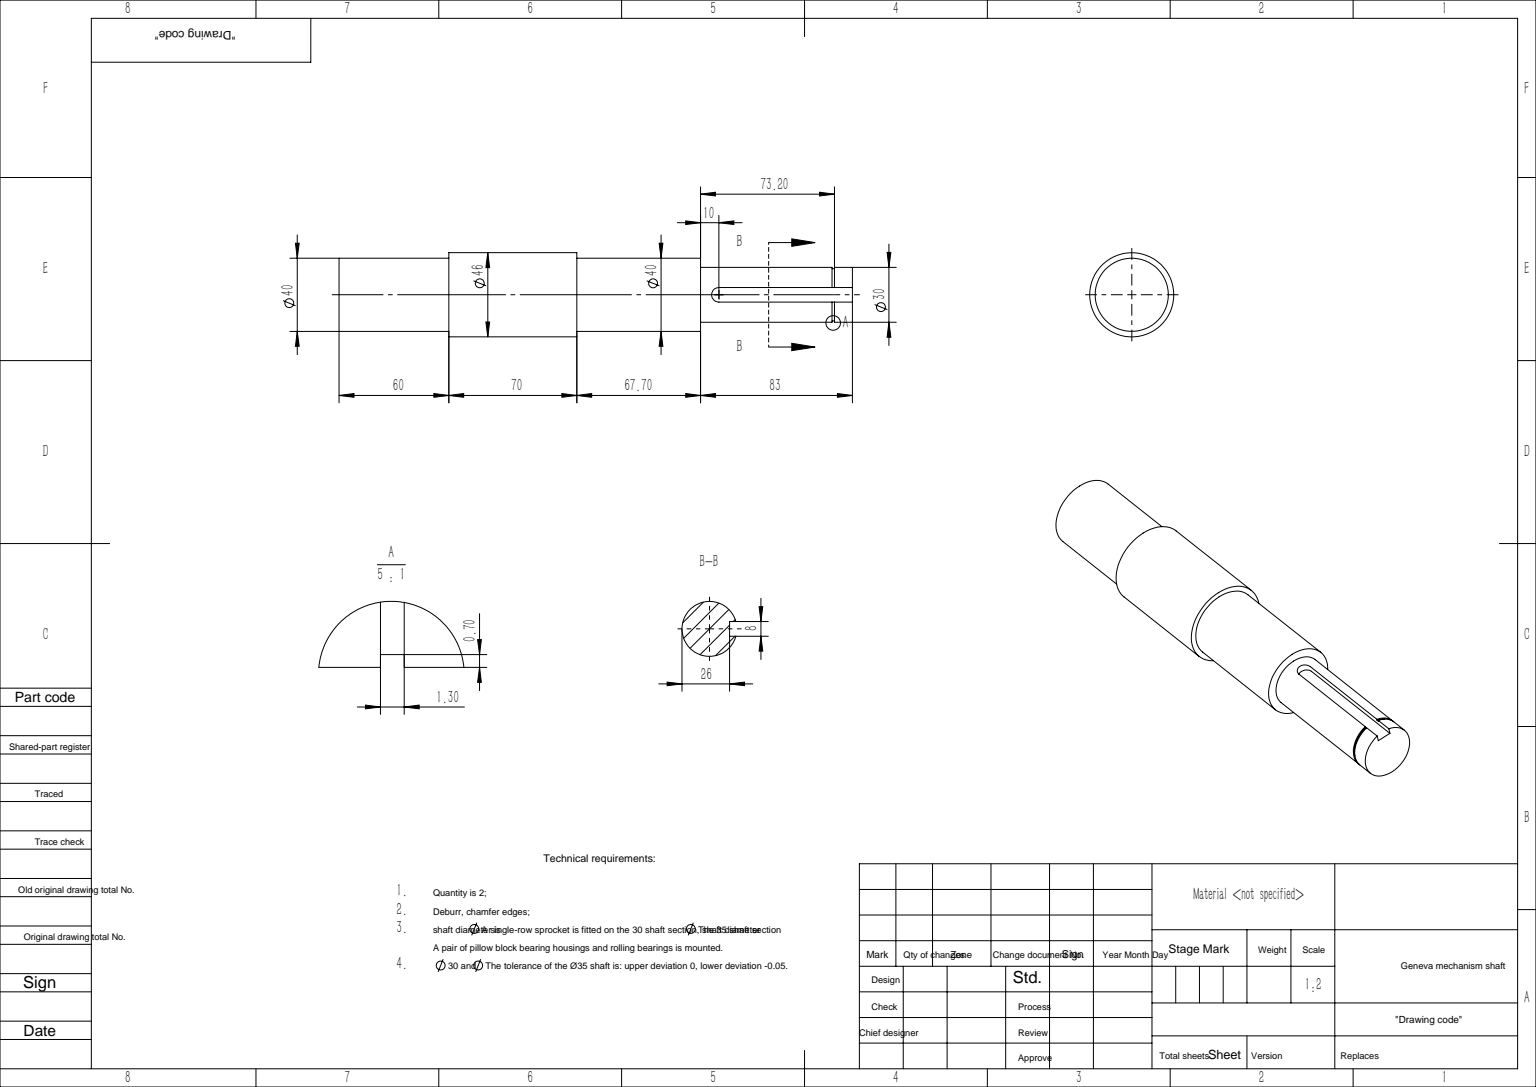
from build123d import *

# Parameters (mm, degrees)
CUT_EXTRUDE_1_DEPTH = 4
SKETCH_3_R          = 15
SKETCH_3_R_2        = 14.3
CUT_EXTRUDE_2_DEPTH = 1.3


with BuildPart() as part:
    # 草图1 → 旋转1 (revolve)
    with BuildSketch(Plane.XY):
        Polygon((0, 0), (0, 20), (60, 20), (60, 23), (130, 23), (130, 20), (197.7, 20), (197.7, 15), (280.7, 15), (280.7, 0), align=None)
    revolve(axis=Axis((280.7, 0, 0), (-1, 0, 0)))

    # 草图2 → 切除-拉伸1 (cut)
    with BuildSketch(Plane(origin=(0, 15, 0), x_dir=(1, 0, 0), z_dir=(0, 1, 0))):
        with BuildLine():
            Line((207.7, 4), (290.7, 4))
            Line((290.7, 4), (290.7, -4))
            Line((290.7, -4), (207.7, -4))
            ThreePointArc((207.7, -4), (203.7, 0), (207.7, 4))
        make_face()
    extrude(amount=-CUT_EXTRUDE_1_DEPTH, mode=Mode.SUBTRACT)

    # 草图3 → 切除-拉伸2 (cut)
    with BuildSketch(Plane(origin=(270.9, 0, 0), x_dir=(0, 0, -1), z_dir=(1, 0, 0))):
        with Locations(Location((0, 0, 0), (0, 0, 90))):
            Circle(SKETCH_3_R)
        Circle(SKETCH_3_R_2, mode=Mode.SUBTRACT)
    extrude(amount=-CUT_EXTRUDE_2_DEPTH, mode=Mode.SUBTRACT)


solid = part.part
